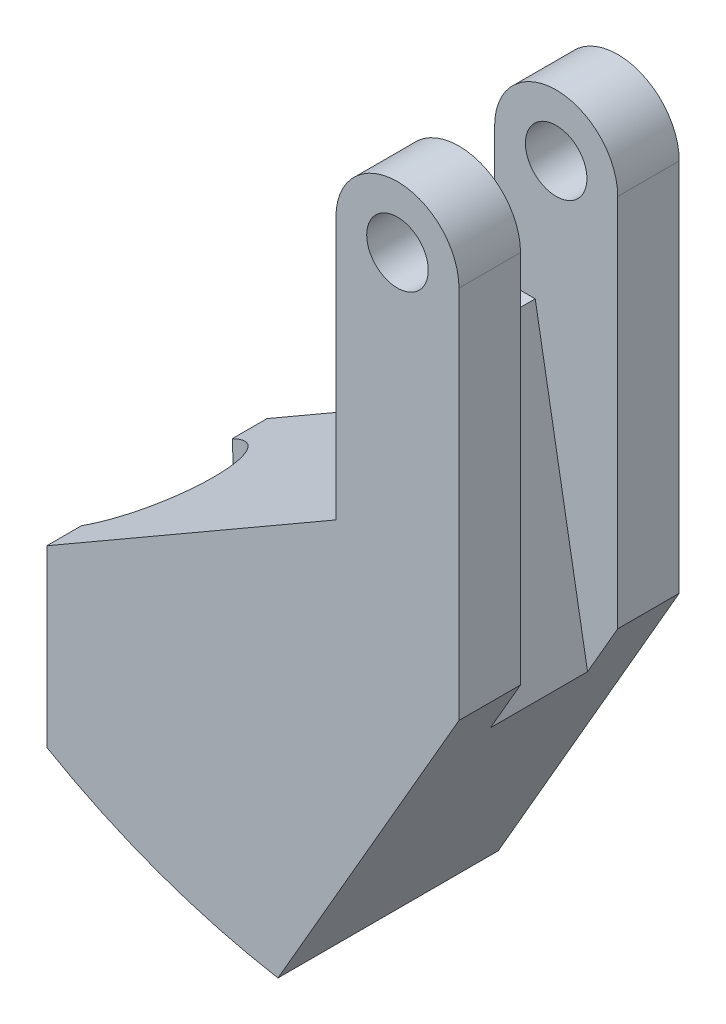
from build123d import *

# Parameters (mm, degrees)
SKETCH2_R           = 2.5
BOSS_EXTRUDE1_DEPTH = 17.9
CUT_EXTRUDE1_DEPTH  = 3.95
SKETCH4_W           = 7.9
SKETCH4_H           = 17.88597718
CUT_EXTRUDE2_DEPTH  = 41.9
SKETCH5_R           = 6.2
CUT_EXTRUDE3_DEPTH  = 41.9


with BuildPart() as part:
    # Sketch2 → Boss-Extrude1 (new body)
    with BuildSketch(Plane.XY):
        with BuildLine():
            Line((5, -30.431019852), (5, 0))
            ThreePointArc((5, 0), (0, 5), (-5, 0))
            Line((-5, 0), (-5, -21.316065276))
            Line((-5, -21.316065276), (-28.5, -34.883796602))
            Line((-28.5, -34.883796602), (-28.5, -49.07456062))
            ThreePointArc((-28.5, -49.07456062), (-19.40948098, -53.327615248), (-9.711912859, -55.9128004))
            Line((-9.711912859, -55.9128004), (5, -30.431019852))
        make_face()
        with Locations(Location((0, 0, 0), (0, 0, 180))):
            Circle(SKETCH2_R, mode=Mode.SUBTRACT)
    extrude(amount=BOSS_EXTRUDE1_DEPTH)

    # Sketch3 → Cut-Extrude1 (cut, symmetric)
    with BuildSketch(Plane(origin=(0, 0, 8.95), x_dir=(-1, 0, 0), z_dir=(0, 0, -1))):
        Polygon((1.84861519, -9.72875797), (-2.55, -34.674544331), (-5, -30.431019852), (-5, -8.521162332), align=None)
    extrude(amount=CUT_EXTRUDE1_DEPTH, both=True, mode=Mode.SUBTRACT)

    # Sketch4 → Cut-Extrude2 (cut)
    with BuildSketch(Plane.ZY.offset(5)):
        with Locations((8.95, -1.613076686)):
            Rectangle(SKETCH4_W, SKETCH4_H)
    extrude(amount=-CUT_EXTRUDE2_DEPTH, mode=Mode.SUBTRACT)

    # Sketch5 → Cut-Extrude3 (cut)
    with BuildSketch(Plane(origin=(19.409643134, -53.32755623, 0), x_dir=(0, 0, -1), z_dir=(0.34202014332566744, -0.9396926207859089, 0))):
        with Locations((-8.95, -39.667670129)):
            Circle(SKETCH5_R)
    extrude(amount=-CUT_EXTRUDE3_DEPTH, mode=Mode.SUBTRACT)


solid = part.part
